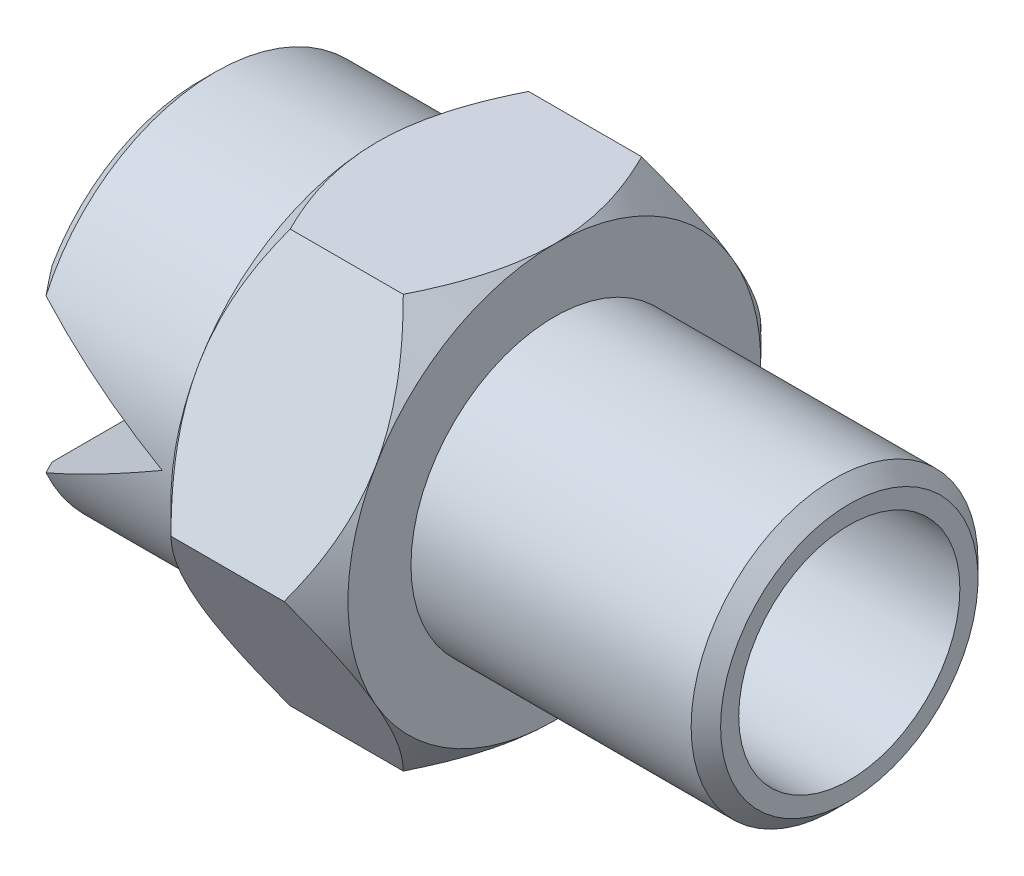
SolidWorks part; units mm, degrees
ref_plane "Front Plane" through (0, 0, 0) normal (0, 0, 1) x (1, 0, 0)
ref_plane "Top Plane" through (0, 0, 0) normal (0, 1, 0) x (1, 0, 0)
ref_plane "Right Plane" through (0, 0, 0) normal (1, 0, 0) x (0, 0, -1)
sketch "Sketch1" plane through (0, 0, 0) normal (0, 0, 1) x (1, 0, 0)
  line L0 (0, 0) -> (50000, 0) construction
  line L1 (0, 0) -> (0, 5.8)
  line L2 (0, 5.8) -> (0.5, 6.3)
  line L3 (0.5, 6.3) -> (6, 6.3)
  line L4 (6, 6.3) -> (6, 7)
  line L5 (6, 7) -> (12, 7)
  line L6 (12, 7) -> (12, 4.864)
  line L7 (12, 4.864) -> (21.5, 4.864)
  line L8 (21.5, 4.864) -> (22, 4.364)
  line L9 (22, 4.364) -> (22, 3.75)
  line L10 (22, 3.75) -> (6, 3.75)
  line L11 (6, 3.75) -> (6, 0)
  line L12 (6, 0) -> (0, 0)
  dimension "D1" = 135
  dimension "D2" = 0.5
  dimension "D3" = 135
  dimension "D4" = 0.5
  dimension "D5" = 7.5
  dimension "D6" = 12.6
  dimension "D7" = 14
  dimension "D8" = 6
  dimension "D9" = 22
  dimension "D10" = 10
  dimension "D11" = 9.728
revolve "Revolve1" add sketch "Sketch1" angle 360 about L0
cosmetic thread "Cosmetic Thread1"
sketch "Sketch2" plane through (12, 0, 0) normal (1, 0, 0) x (0, 0, -1)
  line L1 (8.0829, 0) -> (4.0415, 7)
  line L2 (4.0415, 7) -> (-4.0415, 7)
  line L3 (-4.0415, 7) -> (-8.0829, 0)
  line L4 (-8.0829, 0) -> (-4.0415, -7)
  line L5 (-4.0415, -7) -> (4.0415, -7)
  line L6 (4.0415, -7) -> (8.0829, 0)
  circle A0 centre (0, 0) radius 7 construction
  circle A1 centre (0, 0) radius 7 construction
  circle A2 centre (0, 0) radius 4.864
  circle A3 centre (0, 0) radius 4.864 construction
extrude "Boss-Extrude1" add sketch "Sketch2" against normal up to surface (6 mm away) up to face at (6, 0, 6.3)
sketch "Sketch3" plane through (0, 0, 0) normal (0, 1, 0) x (1, 0, 0)
  line L0 (0, 0) -> (-50000, 0) construction
  line L1 (0, 5.8) -> (0, -5.8) construction
  line L2 (10.9171, 8.0829) -> (12, 7)
  line L3 (6, 8.0829) -> (12, 8.0829) construction
  line L4 (12, 8.0829) -> (12, 4.0415) construction
  line L5 (12, 7) -> (12, 8.0829)
  line L6 (12, 8.0829) -> (10.9171, 8.0829)
  line L8 (6, 7) -> (7.0829, 8.0829)
  line L9 (6, 4.0415) -> (6, 8.0829) construction
  line L10 (7.0829, 8.0829) -> (6, 8.0829)
  line L11 (6, 8.0829) -> (6, 7)
  point P4 (0, 0)
  dimension "D1" = 45
  dimension "D2" = 14
revolve "Cut-Revolve1" cut sketch "Sketch3" angle 360 about L0
sketch "Sketch4" plane through (0, 0, 0) normal (0, 0, 1) x (1, 0, 0)
  line L0 (0, 0) -> (-50000, 0) construction
  line L1 (0, 5.8) -> (0, -5.8) construction
  line L2 (0, 2.8868) -> (5, 0)
  line L3 (5, 0) -> (0, -2.8868)
  line L4 (0, -2.8868) -> (0, 2.8868)
  point P4 (0, 0)
  dimension "D1" = 60
  dimension "D2" = 5
extrude "Cut-Extrude1" cut sketch "Sketch4" against normal through all and the other way through all
sketch "Sketch5" plane through (6, 0, 0) normal (1, 0, 0) x (0, 0, -1)
  circle A0 centre (0, 0) radius 2.5
  dimension "D1" = 5
extrude "Cut-Extrude2" cut sketch "Sketch5" against normal through all
